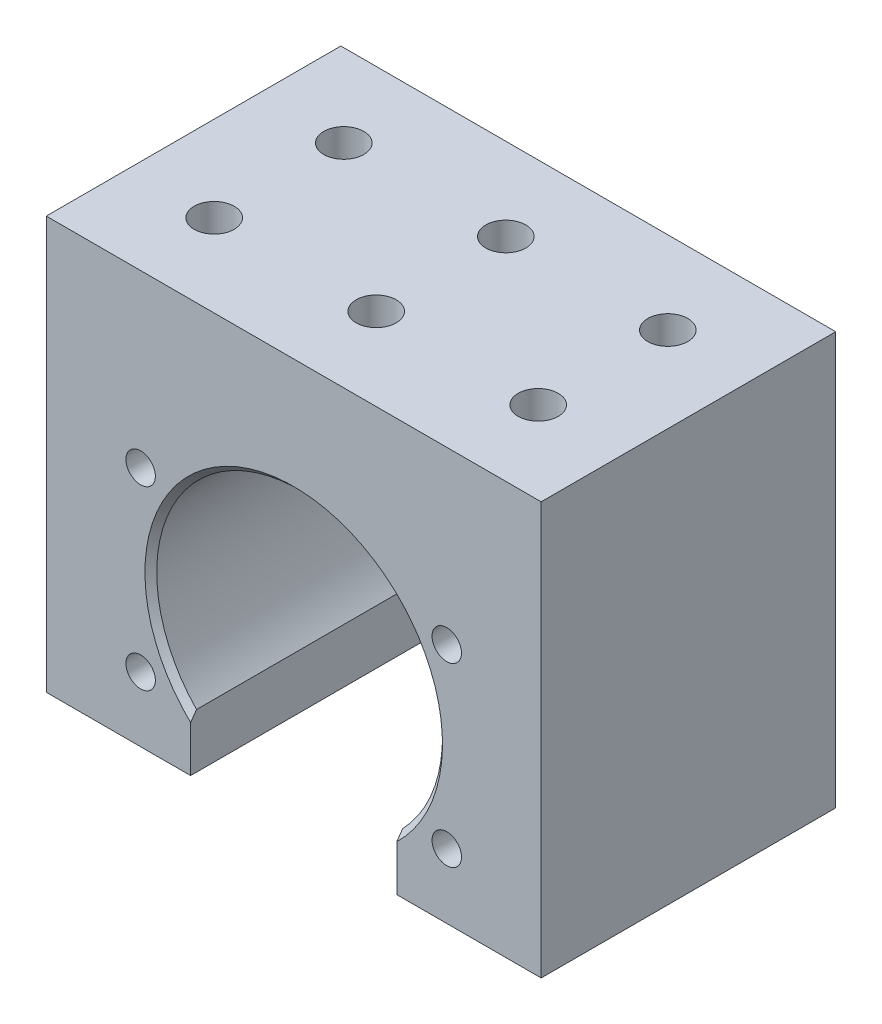
SolidWorks part; units mm, degrees
material "6061Al"
ref_plane "前视基准面" through (0, 0, 0) normal (0, 0, 1) x (1, 0, 0)
ref_plane "上视基准面" through (0, 0, 0) normal (0, 1, 0) x (1, 0, 0)
ref_plane "右视基准面" through (0, 0, 0) normal (1, 0, 0) x (0, 0, -1)
sketch "草图1" plane through (0, 0, 0) normal (0, 0, 1) x (1, 0, 0)
  line L1 (-42, -35) -> (42, -35)
  line L2 (-42, -35) -> (-42, 35)
  line L3 (-42, 35) -> (42, 35)
  line L4 (42, -35) -> (42, 35)
  line L5 (-42, -35) -> (42, 35) construction
  line L6 (-42, 35) -> (42, -35) construction
  circle A0 centre (0, -9) radius 24.25
  point P0 (0, 0)
  dimension "D4" = 48.5
  dimension "D1" = 84
  dimension "D2" = 70
extrude "凸台-拉伸1" add sketch "草图1" along normal mid plane 50
sketch "草图2" plane through (0, 0, 25) normal (0, 0, 1) x (1, 0, 0)
  line L0 (0, 0) -> (0, -35) construction
  line L1 (-42, -35) -> (42, -35) construction
  line L3 (-17.5, -25.7873) -> (17.5, -25.7873)
  line L4 (-17.5, -25.7873) -> (-17.5, -35)
  line L5 (-17.5, -35) -> (17.5, -35)
  line L6 (17.5, -25.7873) -> (17.5, -35)
  circle A0 centre (0, -9) radius 24.25 construction
  dimension "D1" = 35
extrude "切除-拉伸1" cut sketch "草图2" against normal through all
hole_wizard "M6 螺纹孔1" positions "草图3" profile "草图5" tap size "M6" standard "ISO" end condition through all
sketch "草图3" plane through (0, 0, -25) normal (0, 0, -1) x (-1, 0, 0)
  point P0 (-25.9808, 6)
  point P3 (25.9808, 6)
  point P6 (25.9808, -24)
  point P9 (-25.9808, -24)
sketch "草图5" plane through (25.9808, 6, -25) normal (1, 0, 0) x (0, 1, 0)
  line L0 (0, 0) -> (0, 50)
  line L1 (0, 50) -> (2.5, 50)
  line L2 (2.5, 50) -> (2.5, 0)
  line L5 (2.5, 0) -> (0, 0)
  line L11 (0, -6.35) -> (0, 107.95) construction
  dimension "通孔螺纹孔钻头直径" = 5
  dimension "通孔螺纹孔钻头深度" = 50
cosmetic thread "孔螺蚊线1" parameters "D2"=6
cosmetic thread "孔螺蚊线2" parameters "D2"=6
cosmetic thread "孔螺蚊线3" parameters "D2"=6
cosmetic thread "孔螺蚊线4" parameters "D2"=6
hole_wizard "M8 螺纹孔1" positions "草图6" profile "草图7" tap size "M8" standard "ISO"
sketch "草图6" plane through (0, 35, 0) normal (0, 1, 0) x (1, 0, 0)
  line L0 (0, 0) -> (-42, 0) construction
  line L1 (-42, -25) -> (-42, 25) construction
  line L3 (0, 0) -> (0, 25) construction
  line L4 (42, 25) -> (-42, 25) construction
  point P0 (-27.5, 11)
  point P2 (-27.5, -11)
  point P19 (27.5, -11)
  point P20 (27.5, 11)
  point P21 (0, 11)
  point P23 (0, -11)
  dimension "D1" = 22
  dimension "D2" = 55
sketch "草图7" plane through (-27.5, 35, -11) normal (1, 0, 0) x (0, 0, 1)
  line L0 (0, 0) -> (0, 21.7929)
  line L1 (0, 21.7929) -> (3.4, 19.75)
  line L2 (3.4, 19.75) -> (3.4, 0)
  line L5 (3.4, 0) -> (0, 0)
  line L10 (0, 21.7929) -> (-3.4, 19.75) construction
  line L11 (0, -6.35) -> (0, 107.95) construction
  dimension "螺纹孔钻头直径" = 6.8
  dimension "螺纹孔钻头深度" = 19.75
  dimension "导头角度" = 118
cosmetic thread "孔螺蚊线5" parameters "D1"=16, "D2"=8
cosmetic thread "孔螺蚊线6" parameters "D1"=16, "D2"=8
cosmetic thread "孔螺蚊线7" parameters "D1"=16, "D2"=8
cosmetic thread "孔螺蚊线8" parameters "D1"=16, "D2"=8
cosmetic thread "孔螺蚊线9" parameters "D1"=16, "D2"=8
cosmetic thread "孔螺蚊线10" parameters "D1"=16, "D2"=8
chamfer "倒角1" [suppressed] distance 2 angle 45
chamfer "倒角2" distance 1 angle 45 2 edges at (0, 15.25, 25) (0, 15.25, -25)
sketch "草图8" plane through (0, 0, 25) normal (0, 0, 1) x (1, 0, 0)
  line L0 (0, 0) -> (0, 44.1289) construction
  line L1 (102, 35) -> (102, 20)
  line L2 (-42, 35) -> (-102, 35)
  line L3 (-42, 35) -> (-42, 20)
  line L4 (-42, 20) -> (-102, 20)
  line L5 (-102, 35) -> (-102, 20)
  line L6 (42, 20) -> (102, 20)
  line L7 (42, 35) -> (42, 20)
  line L8 (42, 35) -> (102, 35)
  dimension "D1" = 60
  dimension "D2" = 15
extrude "凸台-拉伸2" [suppressed] add sketch "草图8" against normal through all
sketch "草图9" [suppressed] plane through (0, 0, 30) normal (0, 0, 1) x (1, 0, 0)
  line L0 (-42, 20) -> (-42, -35) construction
  line L1 (-102, 20) -> (-50, 20)
  line L2 (-102, 20) -> (-102, -15)
  line L3 (-102, -15) -> (-50, -15)
  line L4 (-50, 20) -> (-50, -15)
  line L5 (0, 0) -> (0, 59.661) construction
  line L6 (50, 20) -> (50, -15)
  line L7 (102, -15) -> (50, -15)
  line L8 (102, 20) -> (102, -15)
  line L9 (102, 20) -> (50, 20)
  dimension "D1" = 8
  dimension "D2" = 35
extrude "凸台-拉伸3" [suppressed] add sketch "草图9" against normal through all
sketch "草图10" [suppressed] plane through (0, 0, 30) normal (0, 0, 1) x (1, 0, 0)
  line L0 (102, 35) -> (-102, 35) construction
  line L1 (-68, 35) -> (-76, 35)
  line L2 (-68, 35) -> (-68, 5)
  line L3 (-68, 5) -> (-76, 5)
  line L4 (-76, 35) -> (-76, 5)
  line L5 (-50, -15) -> (-50, 20) construction
  line L6 (0, 0) -> (0, 65.1966) construction
  line L7 (76, 35) -> (76, 5)
  line L8 (68, 5) -> (76, 5)
  line L9 (68, 35) -> (68, 5)
  line L10 (68, 35) -> (76, 35)
  line L11 (-102, -15) -> (-50, -15) construction
  dimension "D1" = 8
  dimension "D2" = 18
  dimension "D3" = 20
extrude "切除-拉伸2" [suppressed] cut sketch "草图10" against normal through all
sketch "草图12" [suppressed] plane through (0, 0, 30) normal (0, 0, 1) x (1, 0, 0)
  line L0 (68, 35) -> (68, 5) construction
  line L1 (-68, 35) -> (68, 35)
  line L2 (-68, 35) -> (-68, 28)
  line L3 (-68, 28) -> (68, 28)
  line L4 (68, 35) -> (68, 28)
  dimension "D1" = 7
extrude "切除-拉伸3" [suppressed] cut sketch "草图12" against normal through all
